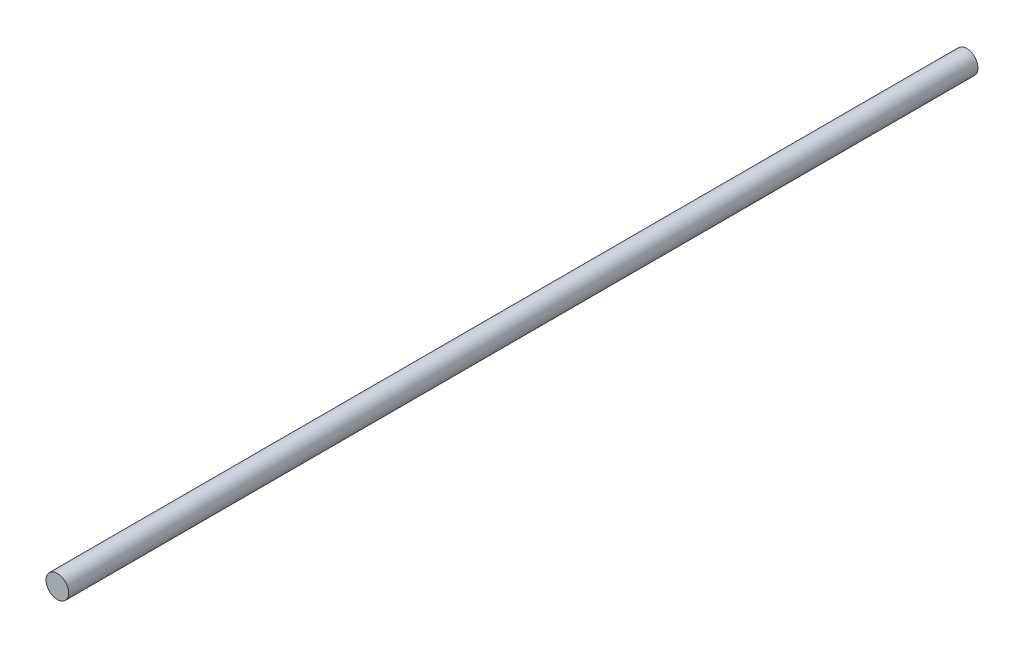
SolidWorks part; units mm, degrees
material "1060 合金"
ref_plane "前视基准面" through (0, 0, 0) normal (0, 0, 1) x (1, 0, 0)
ref_plane "上视基准面" through (0, 0, 0) normal (0, 1, 0) x (1, 0, 0)
ref_plane "右视基准面" through (0, 0, 0) normal (1, 0, 0) x (0, 0, -1)
other "Configuration Table"
sketch "草图1" plane through (0, 0, 0) normal (0, 0, 1) x (1, 0, 0)
  circle A0 centre (0, 0) radius 5
  dimension "D1" = 10
extrude "凸台-拉伸1" add sketch "草图1" along normal blind 400
